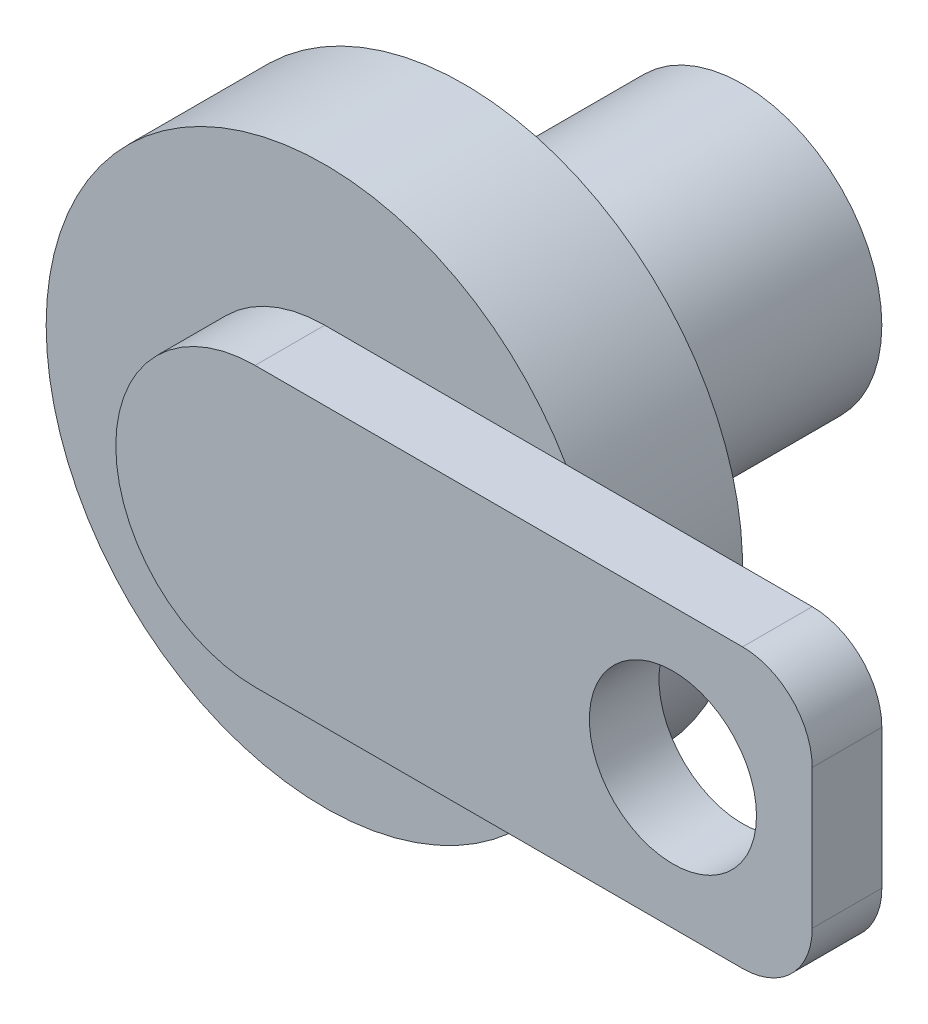
from build123d import *

# Parameters (mm, degrees)
SKETCH1_W           = 100
SKETCH1_H           = 40
BOSS_EXTRUDE1_DEPTH = 10
SKETCH2_R           = 12
CUT_EXTRUDE1_DEPTH  = 10
FILLET1_R           = 10
CUT_EXTRUDE2_DEPTH  = 10
BOSS_EXTRUDE2_START = 60
SKETCH4_R           = 20
BOSS_EXTRUDE2_DEPTH = 60
SKETCH5_R           = 40
BOSS_EXTRUDE3_DEPTH = 20


with BuildPart() as part:
    # Sketch1 → Boss-Extrude1 (new body)
    with BuildSketch(Plane.XY):
        Rectangle(SKETCH1_W, SKETCH1_H)
    extrude(amount=BOSS_EXTRUDE1_DEPTH)

    # Sketch2 → Cut-Extrude1 (cut)
    with BuildSketch(Plane.XY.offset(10)):
        with Locations((30, 0)):
            Circle(SKETCH2_R)
    extrude(amount=-CUT_EXTRUDE1_DEPTH, mode=Mode.SUBTRACT)

    # Fillet1
    fillet1_edges = [part.edges().sort_by_distance(p)[0] for p in [
        (50, -20, 5),
        (50, 20, 5),
    ]]
    fillet(fillet1_edges, radius=FILLET1_R)

    # Sketch3 → Cut-Extrude2 (cut)
    with BuildSketch(Plane(origin=(0, 0, 0), x_dir=(-1, 0, 0), z_dir=(0, 0, -1))):
        with BuildLine():
            Line((50, 20), (30, 20))
            ThreePointArc((30, 20), (44.142135624, 14.142135624), (50, 0))
            Line((50, 0), (50, 20))
        make_face()
        with BuildLine():
            Line((50, -20), (50, 0))
            ThreePointArc((50, 0), (44.142135624, -14.142135624), (30, -20))
            Line((30, -20), (50, -20))
        make_face()
    extrude(amount=-CUT_EXTRUDE2_DEPTH, mode=Mode.SUBTRACT)

    # Sketch4 → Boss-Extrude2 (add)
    with BuildSketch(Plane(origin=(0, 0, 0), x_dir=(-1, 0, 0), z_dir=(0, 0, -1)).offset(BOSS_EXTRUDE2_START)):
        with Locations((30, 0)):
            Circle(SKETCH4_R)
    extrude(amount=-BOSS_EXTRUDE2_DEPTH)

    # Sketch5 → Boss-Extrude3 (add)
    with BuildSketch(Plane(origin=(0, 0, 0), x_dir=(-1, 0, 0), z_dir=(0, 0, -1))):
        with Locations(Location((30, 0, 0), (0, 0, 210))):
            Circle(SKETCH5_R)
    extrude(amount=BOSS_EXTRUDE3_DEPTH)


solid = part.part
